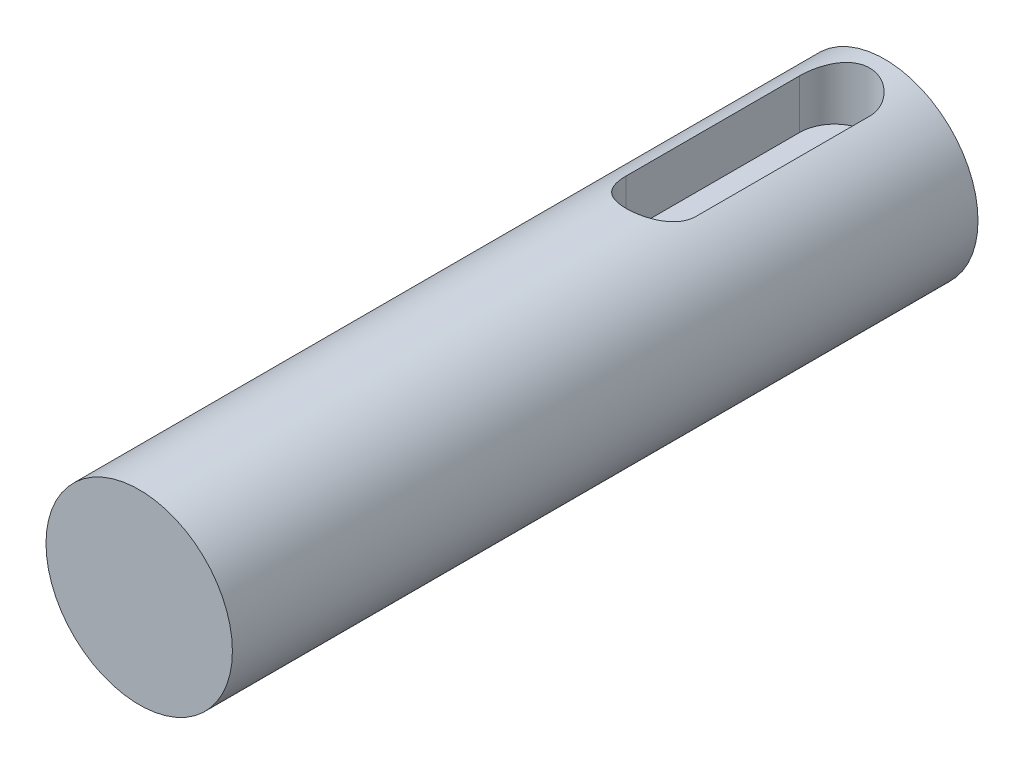
SolidWorks part; units mm, degrees
material "PBT general purpose"
ref_plane "Front Plane" through (0, 0, 0) normal (0, 0, 1) x (1, 0, 0)
ref_plane "Top Plane" through (0, 0, 0) normal (0, 1, 0) x (1, 0, 0)
ref_plane "Right Plane" through (0, 0, 0) normal (1, 0, 0) x (0, 0, -1)
sketch "Sketch1" plane through (0, 0, 0) normal (0, 0, 1) x (1, 0, 0)
  circle A0 centre (0, 0) radius 5
extrude "Boss-Extrude1" add sketch "Sketch1" along normal blind 40
ref_plane "Plane1" through (0, 5, 0) normal (0, 1, 0) x (1, 0, 0)
sketch "Sketch2" plane through (0, 5, 0) normal (0, 1, 0) x (1, 0, 0)
  line L1 (0, -12) -> (0, -2.6916) construction
  line L2 (-1.8768, -12) -> (-1.8768, -2.6916)
  line L3 (1.8768, -12) -> (1.8768, -2.6916)
  arc A0 (-1.8768, -12) -> (1.8768, -12) centre (0, -12) ccw
  arc A1 (1.8768, -2.6916) -> (-1.8768, -2.6916) centre (0, -2.6916) ccw
  point P3 (0, -7.3458)
extrude "Cut-Extrude1" cut sketch "Sketch2" against normal blind 3
